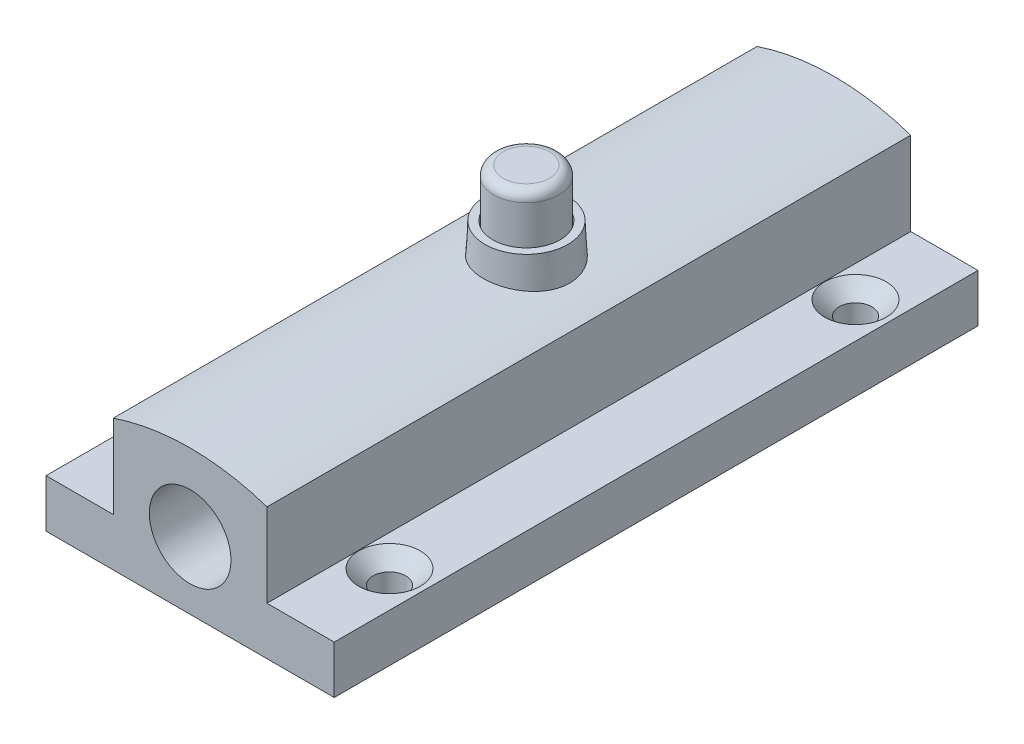
from build123d import *

# Parameters (mm, degrees)
EXTRUDE_1_DEPTH           = 33.5
HOLE_WIZARD_1_D           = 3.4
HOLE_WIZARD_1_CSINK_D     = 6.4
HOLE_WIZARD_1_CSINK_ANGLE = 90
SKETCH_4_R                = 5
EXTRUDE_2_DEPTH           = 13
EXTRUDE_2_TAPER           = 3
SKETCH_6_R                = 3.5
CUT_EXTRUDE_2_DEPTH       = 7
SKETCH_5_R                = 4.25
CUT_EXTRUDE_1_DEPTH       = 71.978870215
SKETCH_7_R                = 3.4
EXTRUDE_3_DEPTH           = 5
FILLET_1_R                = 1


with BuildPart() as part:
    # 草图1 → 凸台-拉伸1 (new, symmetric)
    with BuildSketch(Plane.XY):
        with BuildLine():
            Line((-15, 5), (-8, 5))
            Line((-8, 5), (-8, 13.685438565))
            ThreePointArc((-8, 13.685438565), (0, 15), (8, 13.685438565))
            Line((8, 13.685438565), (8, 5))
            Line((8, 5), (15, 5))
            Line((15, 5), (15, 0))
            Line((15, 0), (-15, 0))
            Line((-15, 0), (-15, 5))
        make_face()
    extrude(amount=EXTRUDE_1_DEPTH, both=True)

    # 打孔尺寸开槽半沉头螺钉的类型1 (through all)
    with Locations(Plane(origin=(0, 5, 0), x_dir=(1, 0, 0), z_dir=(0, 1, 0))):
        with Locations((-11.25, 24.5), (-11.25, -24), (11.25, -24), (11.25, 24.5)):
            CounterSinkHole(HOLE_WIZARD_1_D / 2, HOLE_WIZARD_1_CSINK_D / 2, counter_sink_angle=HOLE_WIZARD_1_CSINK_ANGLE)

    # 草图4 → 凸台-拉伸2 (add)
    with BuildSketch(Plane(origin=(0, 5, 0), x_dir=(1, 0, 0), z_dir=(0, 1, 0))):
        with Locations((0, 1.5)):
            Circle(SKETCH_4_R)
    extrude(amount=EXTRUDE_2_DEPTH, taper=EXTRUDE_2_TAPER)

    # 草图6 → 切除-拉伸2 (cut)
    with BuildSketch(Plane(origin=(0, 18, 0), x_dir=(1, 0, 0), z_dir=(0, 1, 0))):
        with Locations(Location((0, 1.5, 0), (0, 0, 270))):
            Circle(SKETCH_6_R)
    extrude(amount=-CUT_EXTRUDE_2_DEPTH, mode=Mode.SUBTRACT)

    # 草图5 → 切除-拉伸1 (cut, through all)
    with BuildSketch(Plane.XY.offset(33.5)):
        with Locations((0, 7)):
            Circle(SKETCH_5_R)
    extrude(amount=-CUT_EXTRUDE_1_DEPTH, mode=Mode.SUBTRACT)


with BuildPart() as body_2:
    # 草图7 → 凸台-拉伸3 (new, symmetric)
    with BuildSketch(Plane(origin=(0, 18, 0), x_dir=(1, 0, 0), z_dir=(0, 1, 0))):
        with Locations(Location((0, 1.5, 0), (0, 0, 270))):
            Circle(SKETCH_7_R)
    extrude(amount=EXTRUDE_3_DEPTH, both=True)

    # 圆角1
    fillet_1_edges = [body_2.edges().sort_by_distance(p)[0] for p in [
        (0, 23, -4.9),
    ]]
    fillet(fillet_1_edges, radius=FILLET_1_R)


solid = Compound([part.part, body_2.part])
